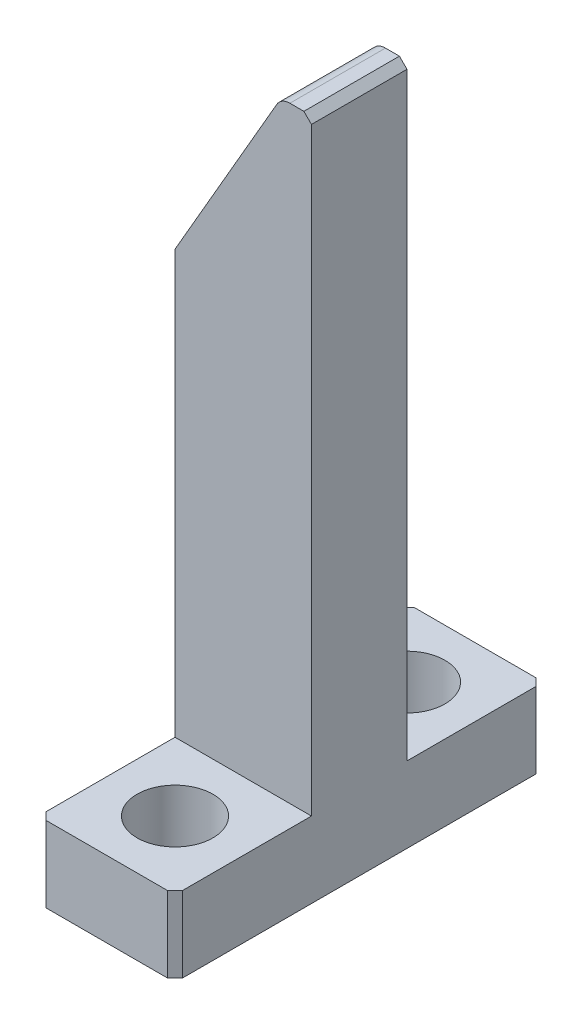
SolidWorks part; units mm, degrees
material "SUJ2"
ref_plane "前视" through (0, 0, 0) normal (0, 0, 1) x (1, 0, 0)
ref_plane "上视" through (0, 0, 0) normal (0, 1, 0) x (1, 0, 0)
ref_plane "右视" through (0, 0, 0) normal (1, 0, 0) x (0, 0, -1)
sketch "草图1" plane through (0, 0, 0) normal (0, 0, 1) x (1, 0, 0)
  line L1 (-4.5, 20) -> (4.5, 20)
  line L2 (-4.5, 20) -> (-4.5, -20)
  line L3 (-4.5, -20) -> (4.5, -20)
  line L4 (4.5, 20) -> (4.5, -20)
  line L5 (-4.5, 20) -> (4.5, -20) construction
  line L6 (-4.5, -20) -> (4.5, 20) construction
  point P0 (0, 0)
  dimension "D1" = 40
  dimension "D2" = 9
extrude "凸台-拉伸1" add sketch "草图1" along normal blind 6.3
sketch "草图2" plane through (0, -20, 0) normal (0, -1, 0) x (1, 0, 0)
  line L1 (-4.5, 6.3) -> (-4.5, 0) construction
  line L2 (-4.5, 15.3) -> (4.5, 15.3)
  line L3 (-4.5, 15.3) -> (-4.5, -9)
  line L4 (-4.5, -9) -> (4.5, -9)
  line L5 (4.5, 15.3) -> (4.5, -9)
  line L6 (4.5, 6.3) -> (4.5, 0) construction
  line L7 (-4.5, 0) -> (4.5, 0) construction
  line L8 (-4.5, 6.3) -> (4.5, 6.3) construction
  dimension "D1" = 0
  dimension "D2" = 0
  dimension "D3" = 9
  dimension "D4" = 9
extrude "凸台-拉伸2" add sketch "草图2" along normal blind 5
sketch "草图3" plane through (0, 0, 0) normal (0, 0, -1) x (-1, 0, 0)
  line L0 (-2.5, 20) -> (4.5, 20)
  line L1 (4.5, 20) -> (4.5, 7.8756)
  line L2 (4.5, 20) -> (4.5, -20) construction
  line L4 (4.5, 7.8756) -> (-2.5, 20)
  dimension "D1" = 7
  dimension "D2" = 60
extrude "切除-拉伸1" cut sketch "草图3" against normal through all
sketch "草图4" plane through (0, -20, 0) normal (0, 1, 0) x (1, 0, 0)
  line L0 (4.5, -6.3) -> (4.5, -15.3) construction
  line L1 (4.5, 9) -> (4.5, 0) construction
  line L2 (-4.5, 9) -> (4.5, 9) construction
  line L3 (4.5, -15.3) -> (-4.5, -15.3) construction
  circle A0 centre (0, 4.5) radius 2.5
  circle A1 centre (0, -10.8) radius 2.5
  dimension "D1" = 5
  dimension "D2" = 5
  dimension "D3" = 4.5
  dimension "D5" = 4.5
  dimension "D4" = 4.5
  dimension "D6" = 4.5
extrude "切除-拉伸2" cut sketch "草图4" against normal through all
chamfer "倒角1" [suppressed] distance 0.5 angle 45
fillet "圆角1" radius 1 1 edges at (2.5, 20, 3.15)
chamfer "倒角2" distance 0.5 angle 45 5 edges at (4.5, -22.5, -9) (-4.5, -22.5, -9) (4.5, -22.5, 15.3) (-4.5, -22.5, 15.3) (4.5, 20, 3.15)
